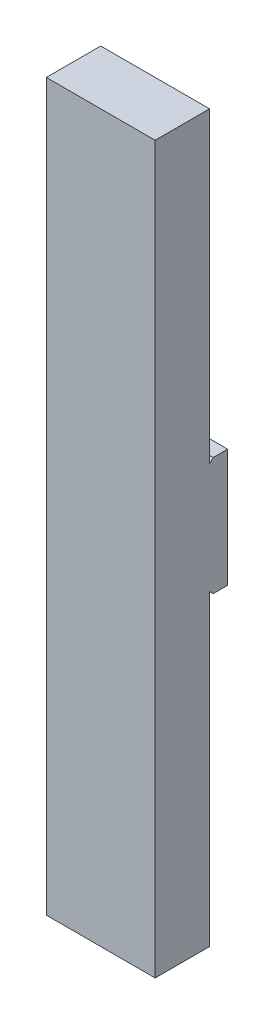
from build123d import *

# Parameters (mm, degrees)
SKETCH_1_W                   = 120
SKETCH_1_H                   = 65
EXTRUDE_1_DEPTH              = 10
CHAMFER_1_SIZE               = 2
SKETCH_2_W                   = 120
SKETCH_2_H                   = 65
EXTRUDE_2_DEPTH              = 30
SKETCH_3_R                   = 10
CUT_EXTRUDE_1_DEPTH          = 2
HOLE_WIZARD_M6_1_D           = 6.6
HOLE_WIZARD_M6_1_CBORE_D     = 13
HOLE_WIZARD_M6_1_CBORE_DEPTH = 35
SKETCH_6_W                   = 60
SKETCH_6_H                   = 400
EXTRUDE_3_DEPTH              = 30
SKETCH_7_W                   = 60
SKETCH_7_H                   = 65
CUT_EXTRUDE_2_DEPTH          = 40


with BuildPart() as part:
    # 草图1 → 凸台-拉伸1 (new body)
    with BuildSketch(Plane.XY):
        Rectangle(SKETCH_1_W, SKETCH_1_H)
    extrude(amount=EXTRUDE_1_DEPTH)

    # 倒角1
    chamfer_1_edges = [part.edges().sort_by_distance(p)[0] for p in [
        (-60, 0, 10),
        (0, -32.5, 10),
        (60, 0, 10),
        (0, 32.5, 10),
    ]]
    chamfer(chamfer_1_edges, length=CHAMFER_1_SIZE)

    # 草图2 → 凸台-拉伸2 (add)
    with BuildSketch(Plane.XY.offset(10)):
        Rectangle(SKETCH_2_W, SKETCH_2_H)
    extrude(amount=EXTRUDE_2_DEPTH)

    # 草图3 → 切除-拉伸1 (cut)
    with BuildSketch(Plane(origin=(0, 0, 0), x_dir=(-1, 0, 0), z_dir=(0, 0, -1))):
        with Locations((-32.5, 0)):
            Circle(SKETCH_3_R)
    extrude(amount=-CUT_EXTRUDE_1_DEPTH, mode=Mode.SUBTRACT)

    # M6 六角头螺栓的柱形沉头孔1 (through all)
    with Locations(Plane.XY.offset(40)):
        with Locations((32.5, 0)):
            CounterBoreHole(HOLE_WIZARD_M6_1_D / 2, HOLE_WIZARD_M6_1_CBORE_D / 2, HOLE_WIZARD_M6_1_CBORE_DEPTH)

    # 草图6 → 凸台-拉伸3 (add)
    with BuildSketch(Plane.XY.offset(40)):
        with Locations((-30, 0)):
            Rectangle(SKETCH_6_W, SKETCH_6_H)
    extrude(amount=-EXTRUDE_3_DEPTH)

    # 草图7 → 切除-拉伸2 (cut)
    with BuildSketch(Plane.XY.offset(40)):
        with Locations((30, 0)):
            Rectangle(SKETCH_7_W, SKETCH_7_H)
    extrude(amount=-CUT_EXTRUDE_2_DEPTH, mode=Mode.SUBTRACT)


solid = part.part
